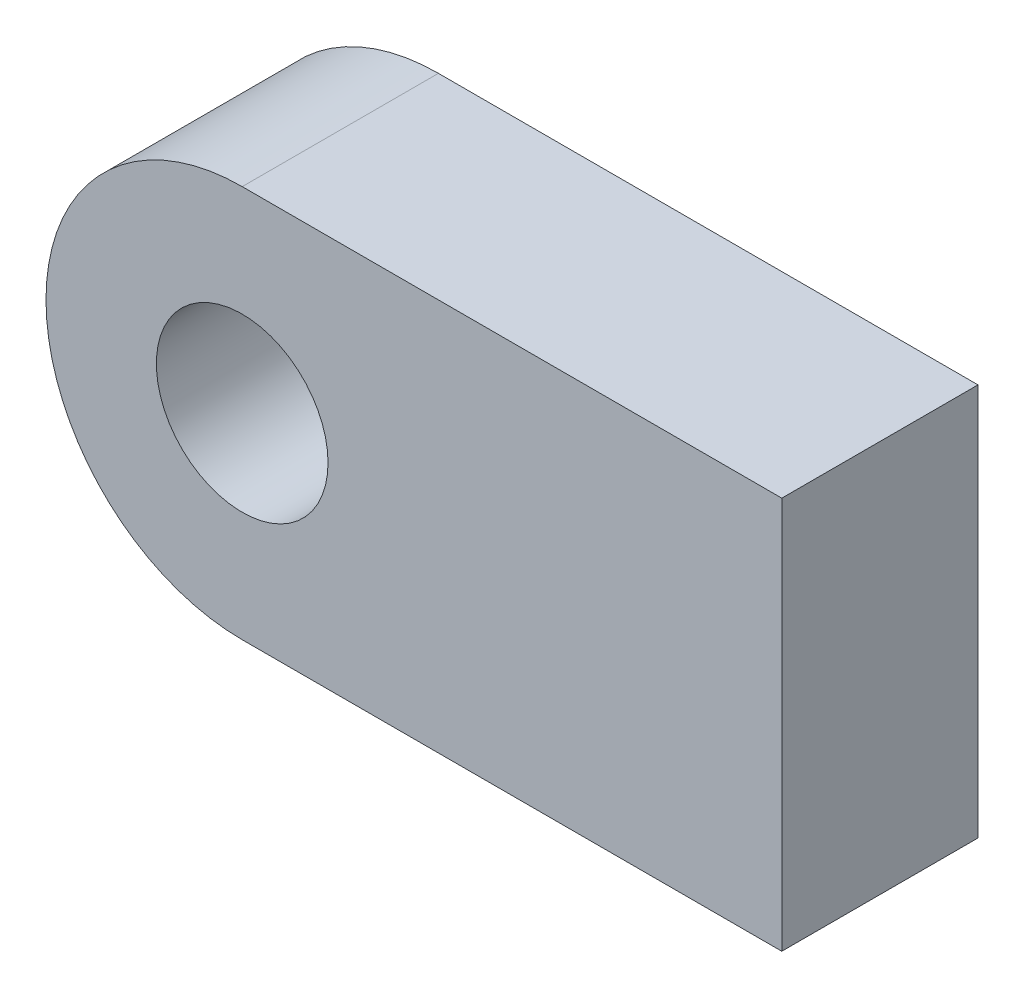
from build123d import *

# Parameters (mm, degrees)
SKETCH1_R           = 3.5
BOSS_EXTRUDE1_DEPTH = 8


with BuildPart() as part:
    # Sketch1 → Boss-Extrude1 (new body)
    with BuildSketch(Plane.XY):
        with BuildLine():
            Line((0, 8), (22, 8))
            Line((22, 8), (22, -8))
            Line((22, -8), (0, -8))
            ThreePointArc((0, -8), (-8, 0), (0, 8))
        make_face()
        Circle(SKETCH1_R, mode=Mode.SUBTRACT)
    extrude(amount=BOSS_EXTRUDE1_DEPTH)


solid = part.part
